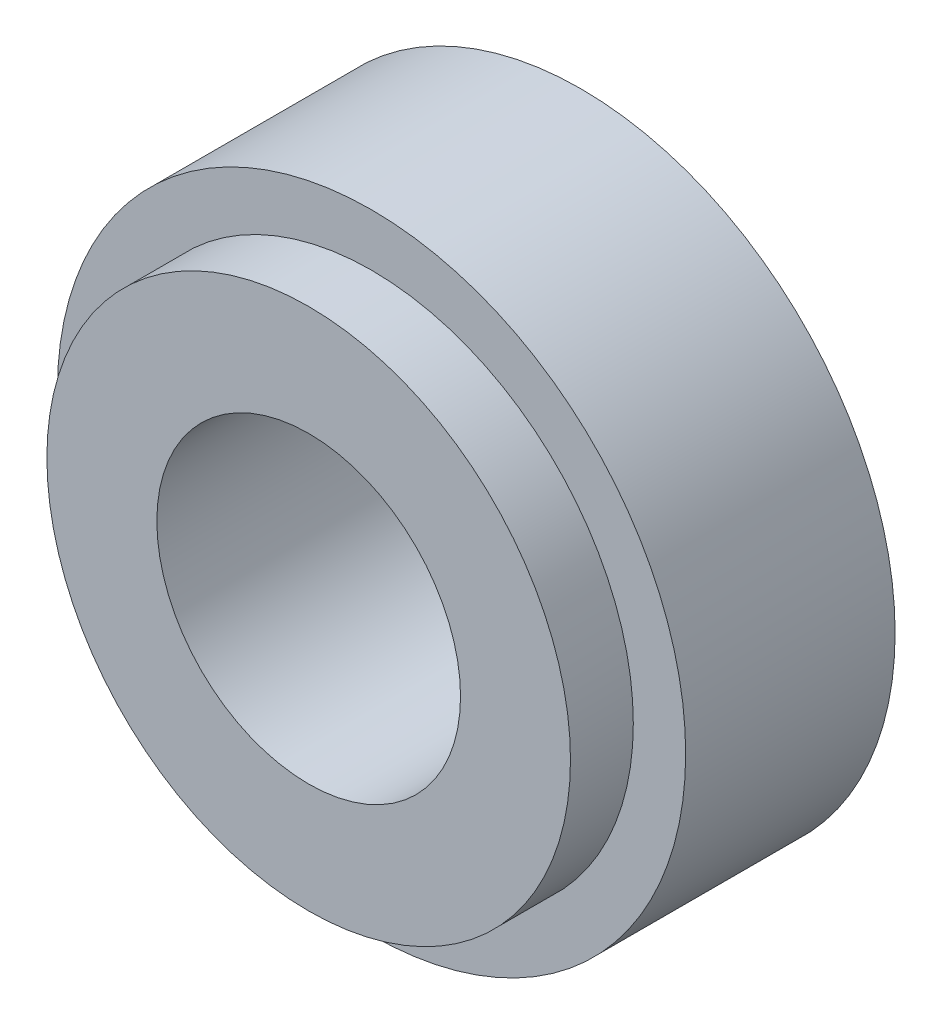
SolidWorks part; units mm, degrees
material "45"
ref_plane "Front Plane" through (0, 0, 0) normal (0, 0, 1) x (1, 0, 0)
ref_plane "Top Plane" through (0, 0, 0) normal (0, 1, 0) x (1, 0, 0)
ref_plane "Right Plane" through (0, 0, 0) normal (1, 0, 0) x (0, 0, -1)
sketch "Sketch1" plane through (0, 0, 0) normal (0, 0, 1) x (1, 0, 0)
  circle A0 centre (0, 0) radius 15
  dimension "D1" = 30
extrude "Boss-Extrude1" add sketch "Sketch1" along normal blind 10
sketch "Sketch2" plane through (0, 0, 10) normal (0, 0, 1) x (1, 0, 0)
  circle A0 centre (0, 0) radius 12.5
  dimension "D1" = 25
extrude "Boss-Extrude2" add sketch "Sketch2" along normal blind 3
sketch "Sketch3" plane through (0, 0, 13) normal (0, 0, 1) x (1, 0, 0)
  circle A0 centre (0, 0) radius 6
  dimension "D1" = 12
extrude "Cut-Extrude1" cut sketch "Sketch3" against normal through all
hole_wizard "M16x1.5 Tapped Hole1" positions "Sketch4" profile "Sketch5" tap size "M16x1.5" standard "GB"
sketch "Sketch4" plane through (0, 0, 0) normal (0, 0, -1) x (-1, 0, 0)
  point P0 (0, 0)
sketch "Sketch5" plane through (0, 0, 0) normal (1, 0, 0) x (0, 1, 0)
  line L0 (0, 0) -> (0, 43.8562)
  line L1 (0, 43.8562) -> (7.25, 39.5)
  line L2 (7.25, 39.5) -> (7.25, 0)
  line L5 (7.25, 0) -> (0, 0)
  line L10 (0, 43.8562) -> (-7.25, 39.5) construction
  line L11 (0, -6.35) -> (0, 107.95) construction
  dimension "螺纹孔钻头直径" = 14.5
  dimension "螺纹孔钻头深度" = 39.5
  dimension "导头角度" = 118
cosmetic thread "Cosmetic thread1" parameters "D1"=13, "D2"=16
